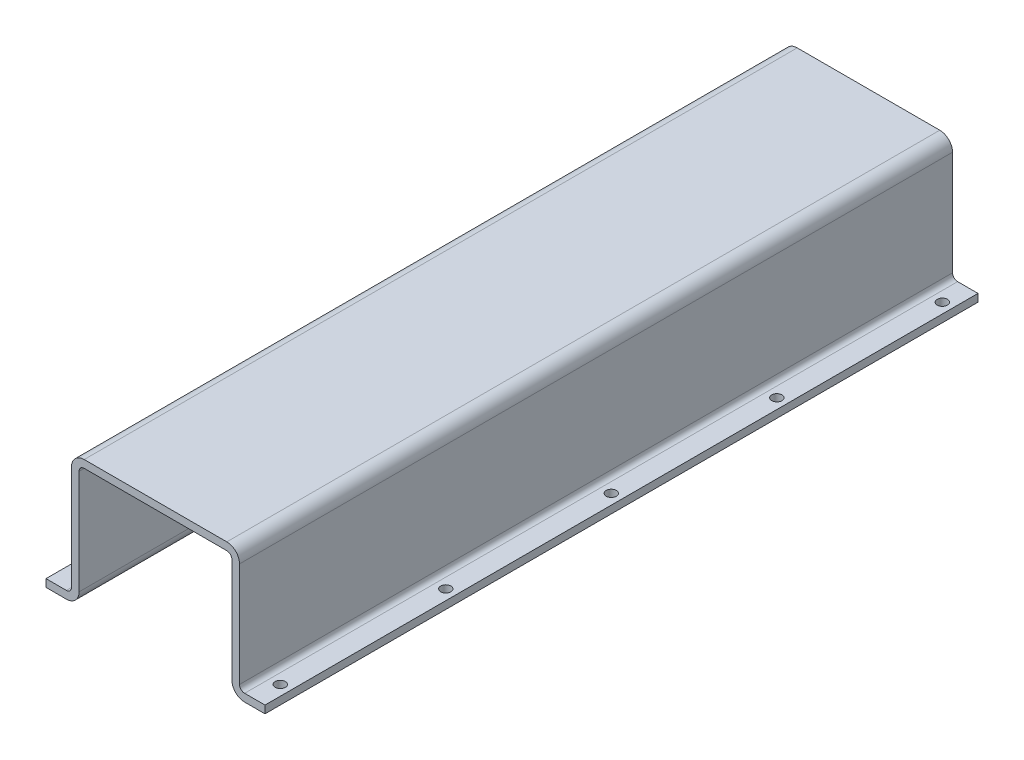
from build123d import *

# Parameters (mm, degrees)
BOSS_EXTRUDE1_DEPTH = 280
SKETCH7_R           = 2
CUT_EXTRUDE3_DEPTH  = 10
LPATTERN1_COUNT     = 5
LPATTERN1_PITCH     = 65


with BuildPart() as part:
    # Sketch1 → Boss-Extrude1 (new body)
    with BuildSketch(Plane.XY):
        with BuildLine():
            Line((86, 0), (86, 3))
            Line((86, 3), (78, 3))
            ThreePointArc((78, 3), (76.585786438, 3.585786438), (76, 5))
            Line((76, 5), (76, 46))
            ThreePointArc((76, 46), (74.535533906, 49.535533906), (71, 51))
            Line((71, 51), (15, 51))
            ThreePointArc((15, 51), (11.464466094, 49.535533906), (10, 46))
            Line((10, 46), (10, 5))
            ThreePointArc((10, 5), (9.414213562, 3.585786438), (8, 3))
            Line((8, 3), (0, 3))
            Line((0, 3), (0, 0))
            Line((0, 0), (8, 0))
            ThreePointArc((8, 0), (11.535533906, 1.464466094), (13, 5))
            Line((13, 5), (13, 46))
            ThreePointArc((13, 46), (13.585786438, 47.414213562), (15, 48))
            Line((15, 48), (71, 48))
            ThreePointArc((71, 48), (72.414213562, 47.414213562), (73, 46))
            Line((73, 46), (73, 5))
            ThreePointArc((73, 5), (74.464466094, 1.464466094), (78, 0))
            Line((78, 0), (86, 0))
        make_face()
    extrude(amount=BOSS_EXTRUDE1_DEPTH)

    # Sketch7 → Cut-Extrude3 (cut)
    with BuildSketch(Plane(origin=(0, 0, 0), x_dir=(-1, 0, 0), z_dir=(0, -1, 0))):
        with Locations(Location((-4, -270, 0), (0, 0, 180))):
            Circle(SKETCH7_R)
        with Locations(Location((-82, -270, 0), (0, 0, 180))):
            Circle(SKETCH7_R)
    cut_extrude3 = extrude(amount=-CUT_EXTRUDE3_DEPTH, mode=Mode.SUBTRACT)

    # LPattern1: Cut-Extrude3 ×5
    with Locations(*[(0, 0, -i * LPATTERN1_PITCH) for i in range(1, LPATTERN1_COUNT)]):
        add(cut_extrude3, mode=Mode.SUBTRACT)


solid = part.part
